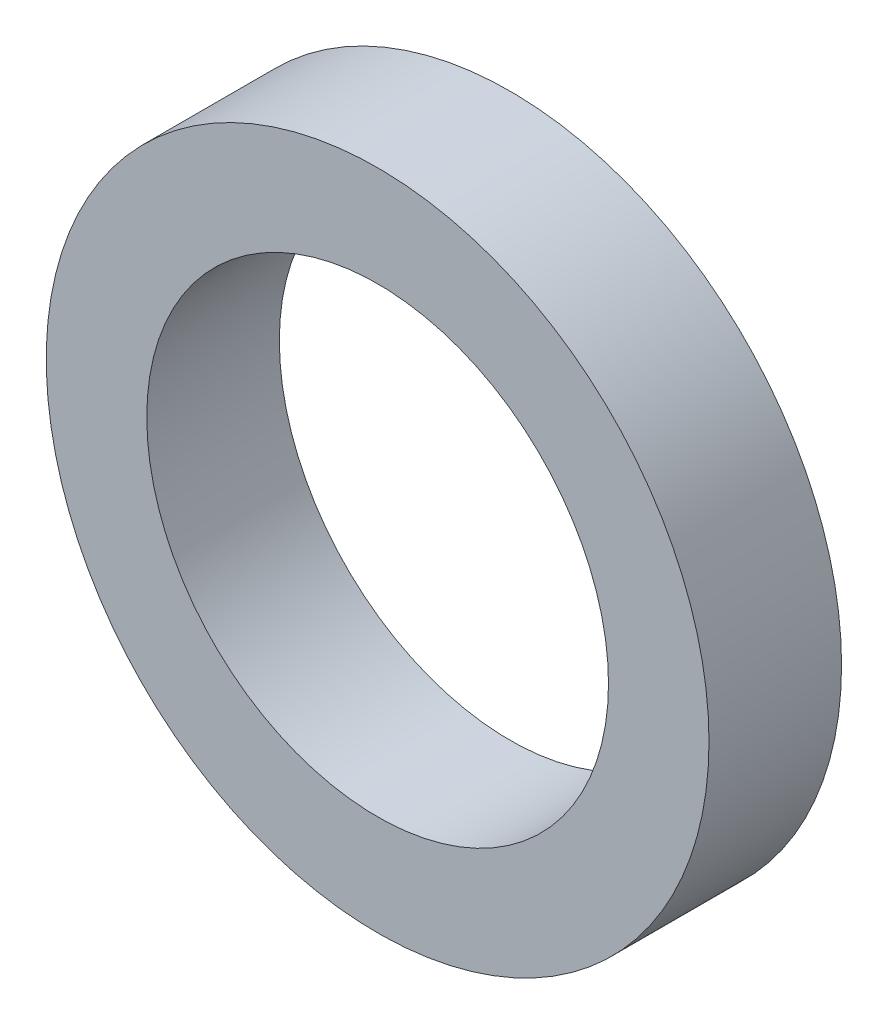
SolidWorks part; units mm, degrees
ref_plane "Front Plane" through (0, 0, 0) normal (0, 0, 1) x (1, 0, 0)
ref_plane "Top Plane" through (0, 0, 0) normal (0, 1, 0) x (1, 0, 0)
ref_plane "Right Plane" through (0, 0, 0) normal (1, 0, 0) x (0, 0, -1)
sketch "Sketch1" plane through (0, 0, 0) normal (0, 0, 1) x (1, 0, 0)
  circle A0 centre (0, 0) radius 30
  circle A1 centre (0, 0) radius 20.9
extrude "Boss-Extrude1" add sketch "Sketch1" along normal blind 12
